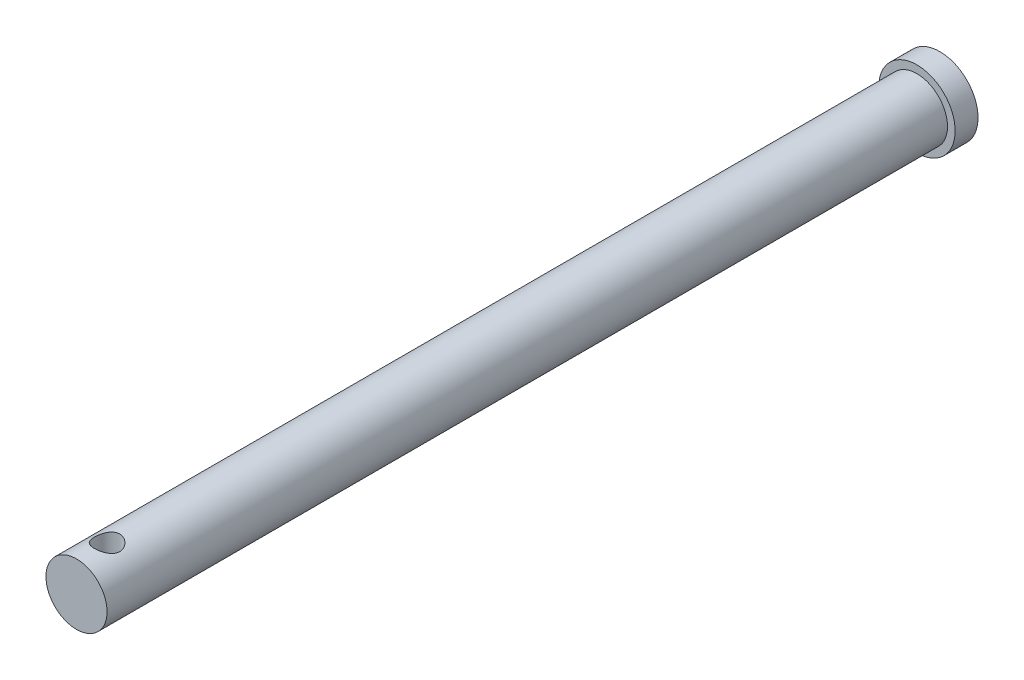
SolidWorks part; units mm, degrees
ref_plane "Front Plane" through (0, 0, 0) normal (0, 0, 1) x (1, 0, 0)
ref_plane "Top Plane" through (0, 0, 0) normal (0, 1, 0) x (1, 0, 0)
ref_plane "Right Plane" through (0, 0, 0) normal (1, 0, 0) x (0, 0, -1)
other "Configuration Table"
sketch "Sketch1" plane through (0, 0, 0) normal (0, 0, 1) x (1, 0, 0)
  circle A0 centre (0, 0) radius 4
  dimension "D1" = 8
extrude "Boss-Extrude1" add sketch "Sketch1" along normal blind 110
sketch "Sketch6" plane through (0, 0, 0) normal (0, 1, 0) x (1, 0, 0)
  line L0 (0, 0) -> (0, -110) construction
  line L1 (-4, -110) -> (4, -110) construction
sketch "Sketch7" plane through (0, 0, 0) normal (0, 0, -1) x (-1, 0, 0)
  circle A0 centre (0, 0) radius 5
  dimension "D1" = 10
extrude "Boss-Extrude2" add sketch "Sketch7" along normal blind 3
sketch "Sketch8" plane through (0, 0, 0) normal (0, 1, 0) x (1, 0, 0)
  line L0 (-4, -110) -> (4, -110) construction
  line L1 (-4, 0) -> (-4, -110) construction
  point P0 (0, -106)
  dimension "D1" = 4
  dimension "D2" = 4
hole_wizard "M4 Tapped Hole1" positions "Sketch8" profile "Sketch9" tap size "M4" standard "GB"
sketch "Sketch9" plane through (0, 0, 106) normal (1, 0, 0) x (0, 0, -1)
  line L0 (0, 0) -> (0, 5)
  line L1 (0, 5) -> (1.65, 5)
  line L2 (1.65, 5) -> (1.65, 0)
  line L5 (1.65, 0) -> (0, 0)
  line L11 (0, -6.35) -> (0, 107.95) construction
  dimension "通孔螺纹孔钻头直径" = 3.3
  dimension "通孔螺纹孔钻头深度" = 5
cosmetic thread "Cosmetic thread 1" parameters "D2"=4
